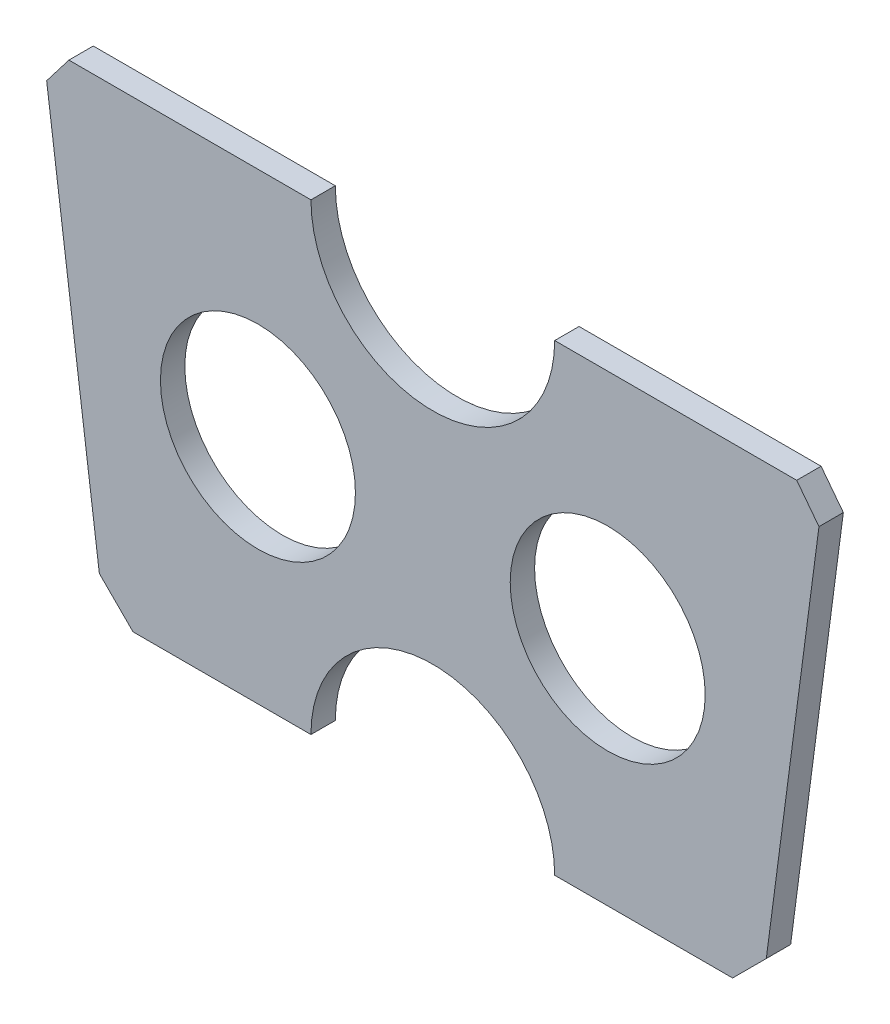
from build123d import *

# Parameters (mm, degrees)
SKETCH1_R           = 40
BOSS_EXTRUDE1_DEPTH = 10


with BuildPart() as part:
    # Sketch1 → Boss-Extrude1 (new body)
    with BuildSketch(Plane.XY):
        with BuildLine():
            Line((149.303943499, 95), (50, 95))
            ThreePointArc((50, 95), (0, 45), (-50, 95))
            Line((-50, 95), (-149.303943499, 95))
            Line((-149.303943499, 95), (-158.434545849, 83.102548453))
            Line((-158.434545849, 83.102548453), (-136.818181818, -81.181818182))
            Line((-136.818181818, -81.181818182), (-123, -95))
            Line((-123, -95), (-50.051564514, -95))
            Line((-50.051564514, -95), (-50, -95))
            ThreePointArc((-50, -95), (0, -45), (50, -95))
            Line((50, -95), (123, -95))
            Line((123, -95), (136.818181818, -81.181818182))
            Line((136.818181818, -81.181818182), (158.434545849, 83.102548453))
            Line((158.434545849, 83.102548453), (149.303943499, 95))
        make_face()
        with Locations((-71.75, 0)):
            Circle(SKETCH1_R, mode=Mode.SUBTRACT)
        with Locations((71.75, 0)):
            Circle(SKETCH1_R, mode=Mode.SUBTRACT)
    extrude(amount=BOSS_EXTRUDE1_DEPTH)


solid = part.part
